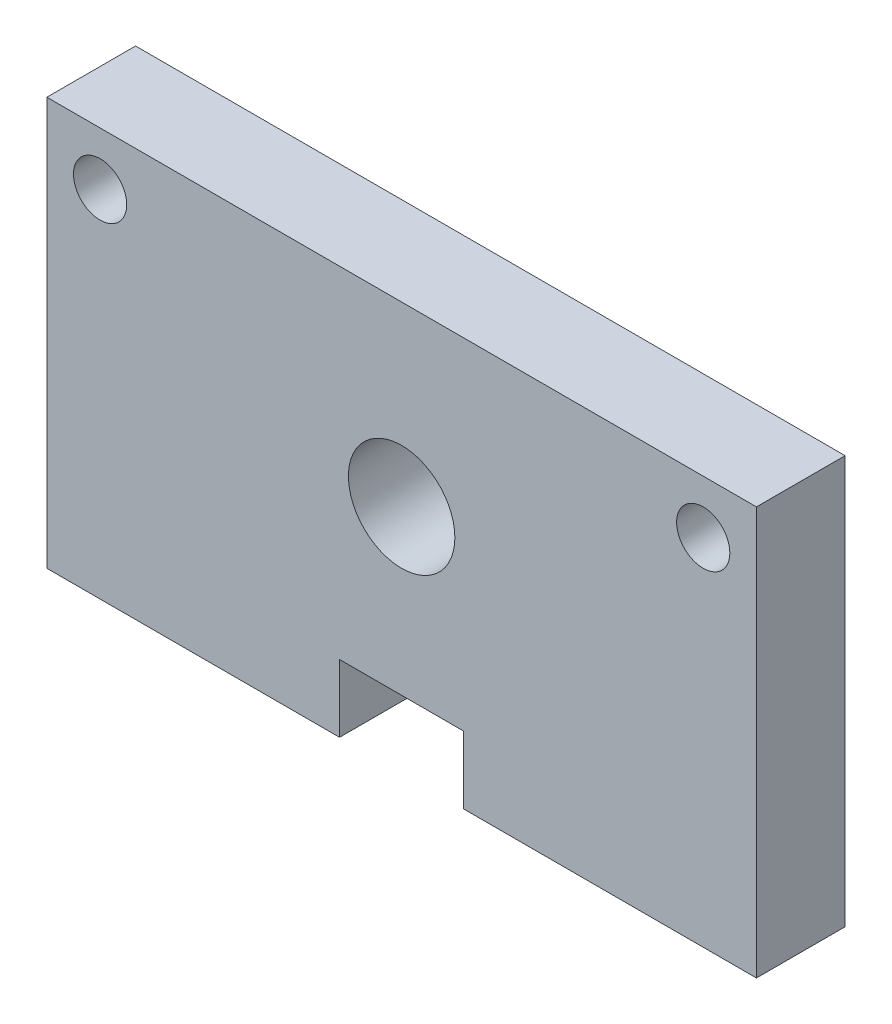
SolidWorks part; units mm, degrees
ref_plane "Front Plane" through (0, 0, 0) normal (0, 0, 1) x (1, 0, 0)
ref_plane "Top Plane" through (0, 0, 0) normal (0, 1, 0) x (1, 0, 0)
ref_plane "Right Plane" through (0, 0, 0) normal (1, 0, 0) x (0, 0, -1)
sketch "Sketch1" plane through (0, 0, 0) normal (0, 0, 1) x (1, 0, 0)
  line L2 (-20, -10) -> (-20, 10)
  line L3 (-20, 10) -> (20, 10)
  line L4 (20, -10) -> (20, 10)
  line L5 (3.5, -13) -> (3.5, -9.2)
  line L9 (20, -10) -> (20, -13)
  line L10 (20, -13) -> (3.5, -13)
  line L11 (-20, -10) -> (-20, -13)
  line L12 (3.5, -9.2) -> (-3.5, -9.2)
  line L13 (-3.5, -9.2) -> (-3.5, -13)
  line L14 (-3.5, -13) -> (-20, -13)
  circle A1 centre (0, 0) radius 3
  circle A2 centre (-17, 7) radius 1.5
  circle A3 centre (17, 7) radius 1.5
  dimension "D1" = 6
  dimension "D2" = 40
  dimension "D4" = 3
  dimension "D5" = 3
  dimension "D6" = 20
  dimension "D9" = 3
  dimension "D3" = 20
  dimension "D8" = 3
  dimension "D12" = 3
  dimension "D13" = 3.8
  dimension "D14" = 7
  dimension "D15" = 3.5
extrude "Boss-Extrude1" add sketch "Sketch1" along normal blind 5
